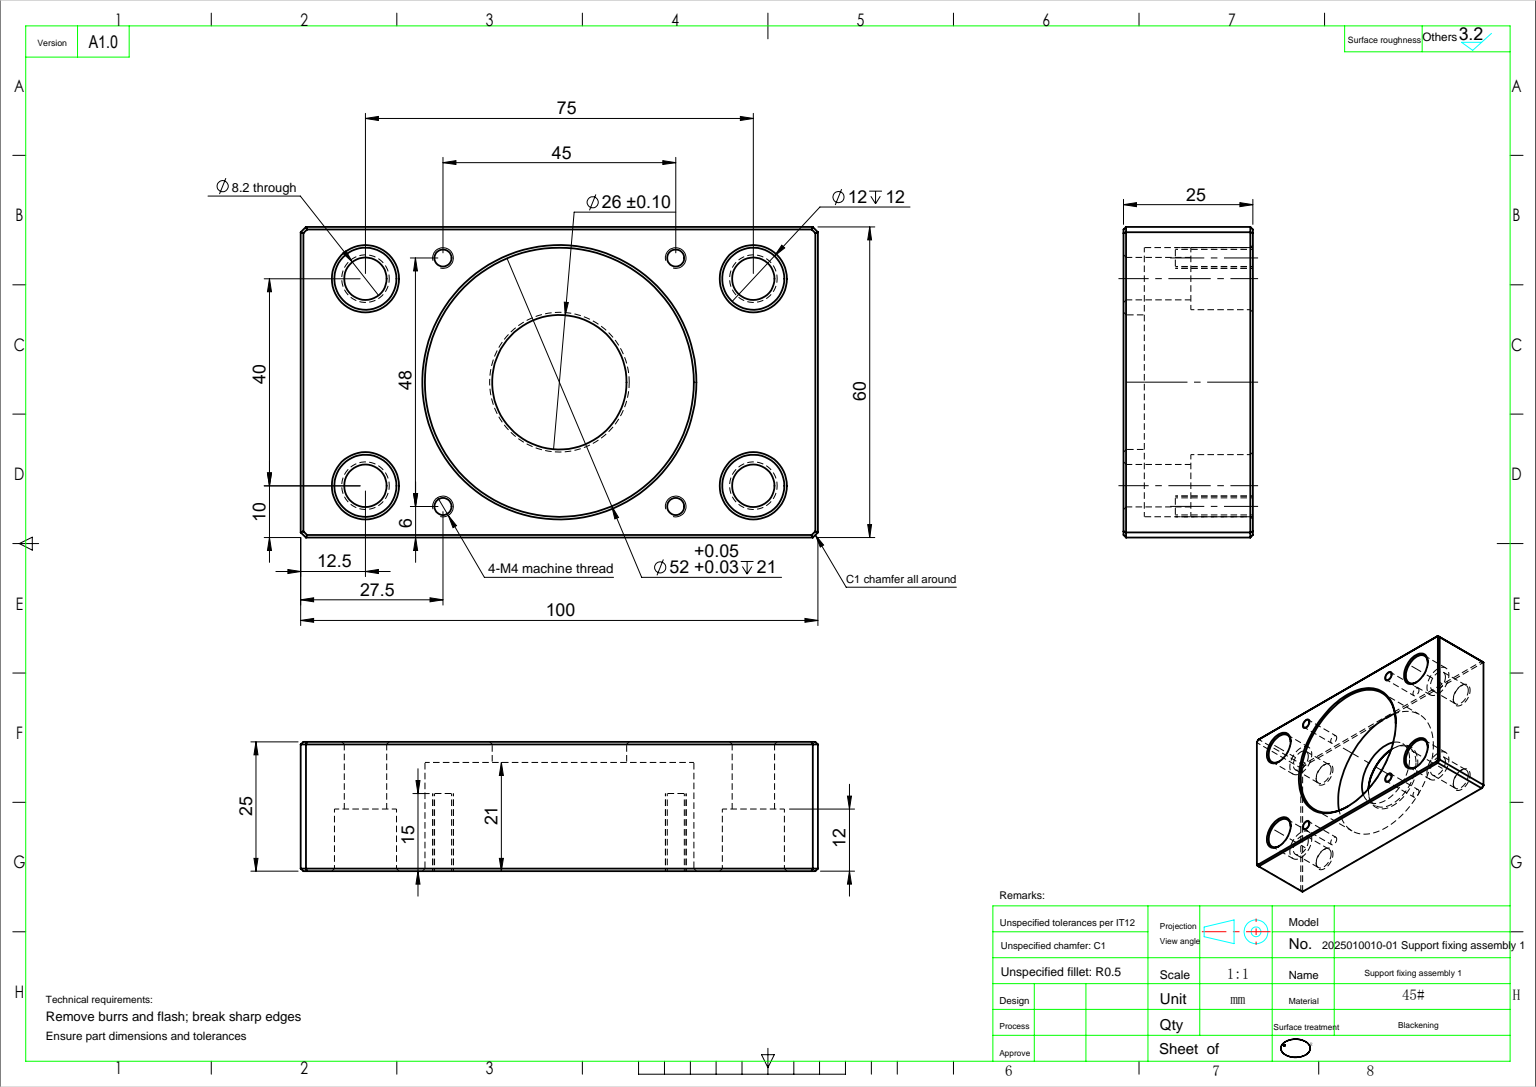
SolidWorks part; units mm, degrees
ref_plane "前视基准面" through (0, 0, 0) normal (0, 0, 1) x (1, 0, 0)
ref_plane "上视基准面" through (0, 0, 0) normal (0, 1, 0) x (1, 0, 0)
ref_plane "右视基准面" through (0, 0, 0) normal (1, 0, 0) x (0, 0, -1)
sketch "草图1" plane through (0, 0, 0) normal (0, 0, 1) x (1, 0, 0)
  line L1 (-50, 30) -> (50, 30)
  line L2 (-50, 30) -> (-50, -30)
  line L3 (-50, -30) -> (50, -30)
  line L4 (50, 30) -> (50, -30)
  line L5 (0, -30) -> (0, 30) construction
  line L6 (-50, 0) -> (50, 0) construction
  point P0 (0, 0)
  dimension "D1" = 60
  dimension "D2" = 100
extrude "凸台-拉伸1" add sketch "草图1" along normal blind 25
sketch "草图2" plane through (0, 0, 25) normal (0, 0, 1) x (1, 0, 0)
  circle A0 centre (0, 0) radius 13
  dimension "D1" = 26
extrude "切除-拉伸1" cut sketch "草图2" against normal through all
sketch "草图3" plane through (0, 0, 25) normal (0, 0, 1) x (1, 0, 0)
  line L1 (-37.5, 20) -> (37.5, 20) construction
  line L2 (-37.5, 20) -> (-37.5, -20) construction
  line L3 (-37.5, -20) -> (37.5, -20) construction
  line L4 (37.5, 20) -> (37.5, -20) construction
  line L5 (0, -20) -> (0, 20) construction
  line L6 (-37.5, 0) -> (37.5, 0) construction
  circle A0 centre (-37.5, 20) radius 6
  circle A1 centre (-37.5, -20) radius 6
  circle A2 centre (37.5, -20) radius 6
  circle A3 centre (37.5, 20) radius 6
  point P0 (0, 0)
  dimension "D3" = 12
  dimension "D1" = 75
  dimension "D2" = 40
extrude "切除-拉伸2" cut sketch "草图3" against normal blind 12
sketch "草图4" plane through (0, 0, 25) normal (0, 0, 1) x (1, 0, 0)
  circle A0 centre (-37.5, 20) radius 4.1
  circle A1 centre (-37.5, -20) radius 4.1
  circle A2 centre (37.5, 20) radius 4.1
  circle A3 centre (37.5, -20) radius 4.1
  dimension "D1" = 8.2
extrude "切除-拉伸3" cut sketch "草图4" against normal through all
chamfer "倒角1" distance 1 angle 45 4 edges at (-50, 30, 12.5) (50, 30, 12.5) (50, -30, 12.5) (-50, -30, 12.5)
chamfer "倒角4" distance 0.5 angle 45 13 edges at (-33.4, -20, 0) (41.6, 20, 0) (41.6, -20, 0) (-33.4, 20, 0) (-49.5, -29.5, 0) (0, -30, 0) (49.5, -29.5, 0) (50, 0, 0) (49.5, 29.5, 0) (0, 30, 0) (-49.5, 29.5, 0) (-50, 0, 0) (13, 0, 0)
sketch "草图8" plane through (0, 0, 25) normal (0, 0, 1) x (1, 0, 0)
  circle A0 centre (0, 0) radius 26
  dimension "D1" = 52
extrude "切除-拉伸5" cut sketch "草图8" against normal blind 21
chamfer "倒角5" distance 0.5 angle 45 13 edges at (49.5, 29.5, 25) (50, 0, 25) (49.5, -29.5, 25) (0, -30, 25) (-49.5, -29.5, 25) (-50, 0, 25) (-49.5, 29.5, 25) (0, 30, 25) (-31.5, 20, 25) (-31.5, -20, 25) (43.5, -20, 25) (43.5, 20, 25) (26, 0, 25)
sketch "草图9" plane through (0, 0, 25) normal (0, 0, 1) x (1, 0, 0)
  line L0 (49, -30) -> (-49, -30) construction
  line L1 (-50, -29) -> (-50, 29) construction
  circle A0 centre (22.5, -24) radius 1.65
  circle A1 centre (22.5, 24) radius 1.65
  circle A2 centre (-22.5, 24) radius 1.65
  circle A3 centre (-22.5, -24) radius 1.65
  dimension "D1" = 3.3
  dimension "D2" = 45
  dimension "D3" = 48
  dimension "D4" = 6
  dimension "D5" = 27.5
extrude "切除-拉伸6" cut sketch "草图9" against normal blind 15
cosmetic thread "装饰螺纹线1" parameters "D2"=4
cosmetic thread "装饰螺纹线2" parameters "D2"=4
cosmetic thread "装饰螺纹线3" parameters "D2"=4
cosmetic thread "装饰螺纹线4" parameters "D2"=4
